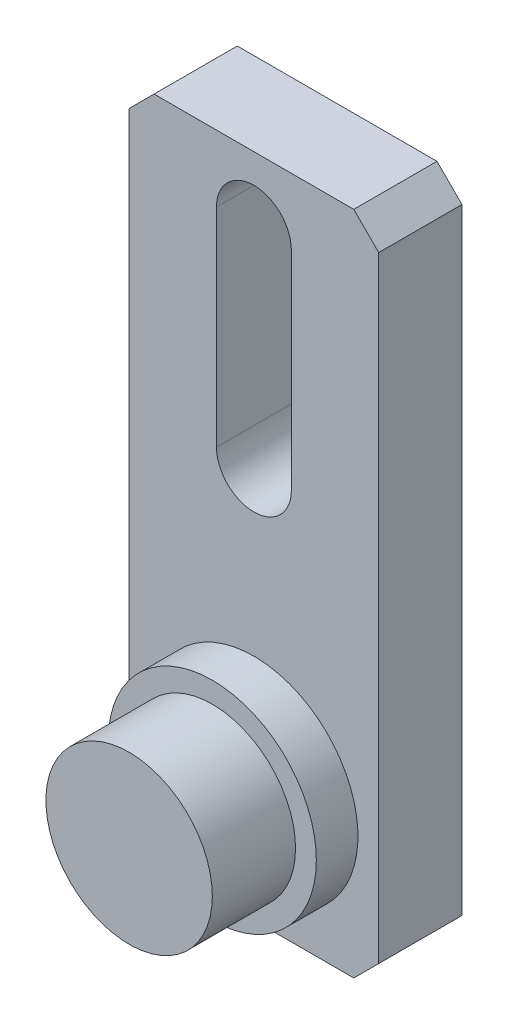
SolidWorks part; units mm, degrees
material "普通碳钢"
ref_plane "前视基准面" through (0, 0, 0) normal (0, 0, 1) x (1, 0, 0)
ref_plane "上视基准面" through (0, 0, 0) normal (0, 1, 0) x (1, 0, 0)
ref_plane "右视基准面" through (0, 0, 0) normal (1, 0, 0) x (0, 0, -1)
sketch "草图1" plane through (0, 0, 0) normal (0, 0, 1) x (1, 0, 0)
  line L1 (-15, -40) -> (15, -40)
  line L2 (-15, -40) -> (-15, 40)
  line L3 (-15, 40) -> (15, 40)
  line L4 (15, -40) -> (15, 40)
  line L5 (-15, -40) -> (15, 40) construction
  line L6 (-15, 40) -> (15, -40) construction
  point P0 (0, 0)
  dimension "D1" = 30
  dimension "D2" = 80
extrude "凸台-拉伸1" add sketch "草图1" along normal blind 10
sketch "草图2" plane through (0, 0, 10) normal (0, 0, 1) x (1, 0, 0)
  line L0 (0, 0) -> (0, -40) construction
  line L1 (-15, -40) -> (15, -40) construction
  circle A0 centre (0, -25) radius 12.5
  dimension "D1" = 25
  dimension "D2" = 15
extrude "凸台-拉伸2" add sketch "草图2" along normal blind 15
sketch "草图3" plane through (0, 0, 25) normal (0, 0, 1) x (1, 0, 0)
  circle A0 centre (0, -25) radius 10
  circle A1 centre (0, -25) radius 12.5 construction
  circle A2 centre (0, -25) radius 12.5
  dimension "D1" = 20
extrude "切除-拉伸1" cut sketch "草图3" against normal blind 10
sketch "草图4" plane through (0, 0, 10) normal (0, 0, 1) x (1, 0, 0)
  line L0 (0, 40) -> (0, 0) construction
  line L1 (15, 40) -> (-15, 40) construction
  line L2 (0, 32) -> (0, 7) construction
  line L3 (4.5, 32) -> (4.5, 7)
  line L4 (-4.5, 32) -> (-4.5, 7)
  arc A0 (4.5, 32) -> (-4.5, 32) centre (0, 32) ccw
  arc A1 (-4.5, 7) -> (4.5, 7) centre (0, 7) ccw
  point P7 (0, 19.5)
  dimension "D1" = 4.5
  dimension "D3" = 8
  dimension "D2" = 25
extrude "切除-拉伸2" cut sketch "草图4" against normal through all
chamfer "倒角1" distance 3 angle 45 4 edges at (-15, -40, 5) (15, -40, 5) (15, 40, 5) (-15, 40, 5)
